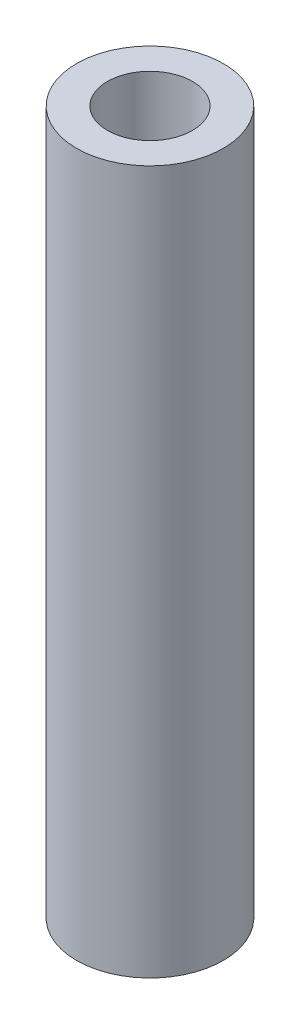
SolidWorks part; units mm, degrees
material "灰铸铁"
ref_plane "前视基准面" through (0, 0, 0) normal (0, 0, 1) x (1, 0, 0)
ref_plane "上视基准面" through (0, 0, 0) normal (0, 1, 0) x (1, 0, 0)
ref_plane "右视基准面" through (0, 0, 0) normal (1, 0, 0) x (0, 0, -1)
other "Configuration Table"
sketch "草图1" plane through (0, 0, 0) normal (0, 1, 0) x (1, 0, 0)
  circle A0 centre (0, 0) radius 9.5
  dimension "D1" = 19
extrude "凸台-拉伸1" add sketch "草图1" along normal blind 91
sketch "草图2" plane through (0, 91, 0) normal (0, 1, 0) x (1, 0, 0)
  circle A0 centre (0, 0) radius 5.5
  dimension "D1" = 11
extrude "切除-拉伸1" cut sketch "草图2" against normal blind 75
hole_wizard "M6 螺纹孔1" positions "草图4" profile "草图5" tap size "M6" standard "GB" end condition through all
sketch "草图4" plane through (0, 0, 0) normal (0, -1, 0) x (1, 0, 0)
  point P0 (0, 0)
sketch "草图5" plane through (0, 0, 0) normal (1, 0, 0) x (0, 0, -1)
  line L0 (0, 0) -> (0, 91)
  line L1 (0, 91) -> (2.5, 91)
  line L2 (2.5, 91) -> (2.5, 0)
  line L5 (2.5, 0) -> (0, 0)
  line L11 (0, -6.35) -> (0, 107.95) construction
  dimension "通孔螺纹孔钻头直径" = 5
  dimension "通孔螺纹孔钻头深度" = 91
cosmetic thread "孔螺纹线2" parameters "D1"=6, "D2"=6
